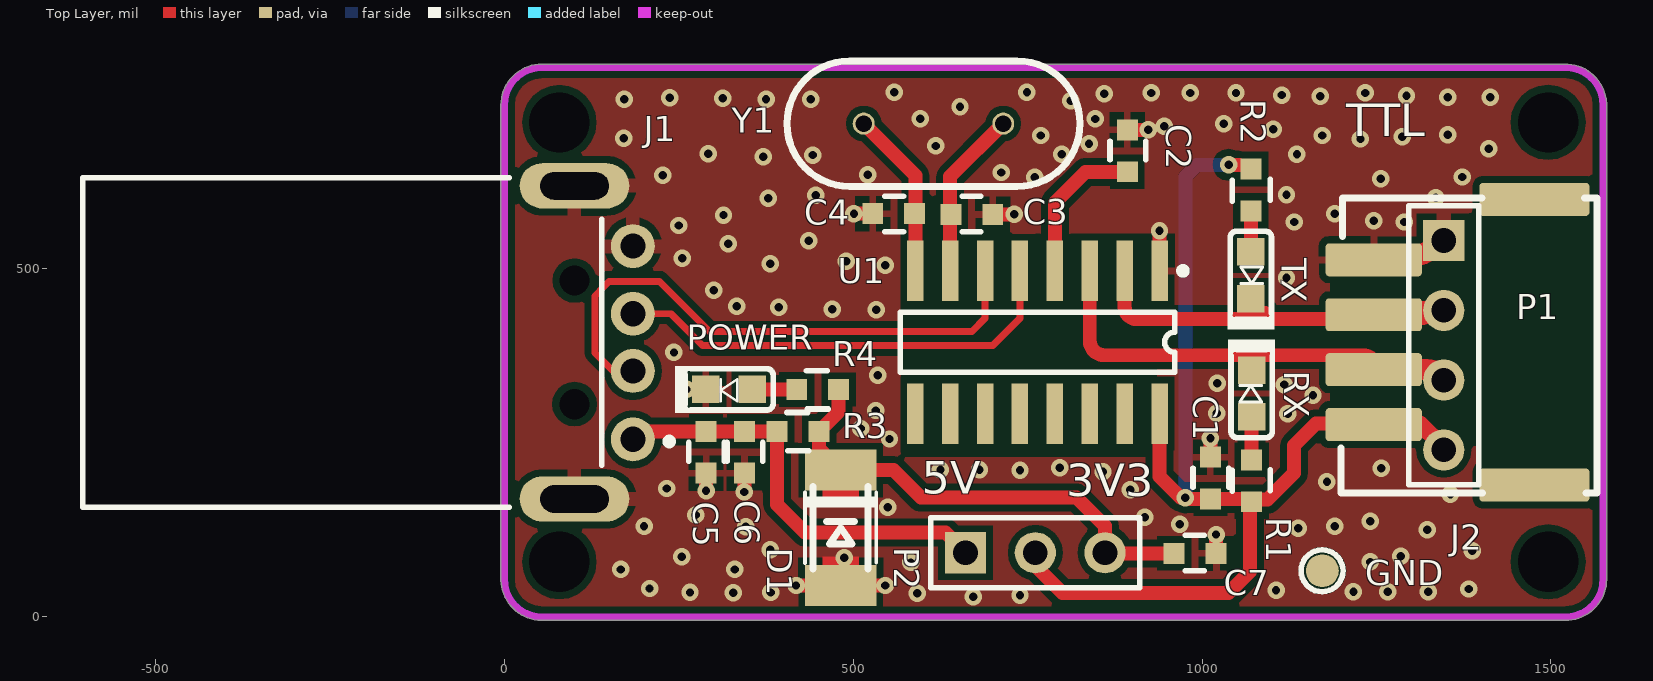
[diagram p0: Top Layer view]
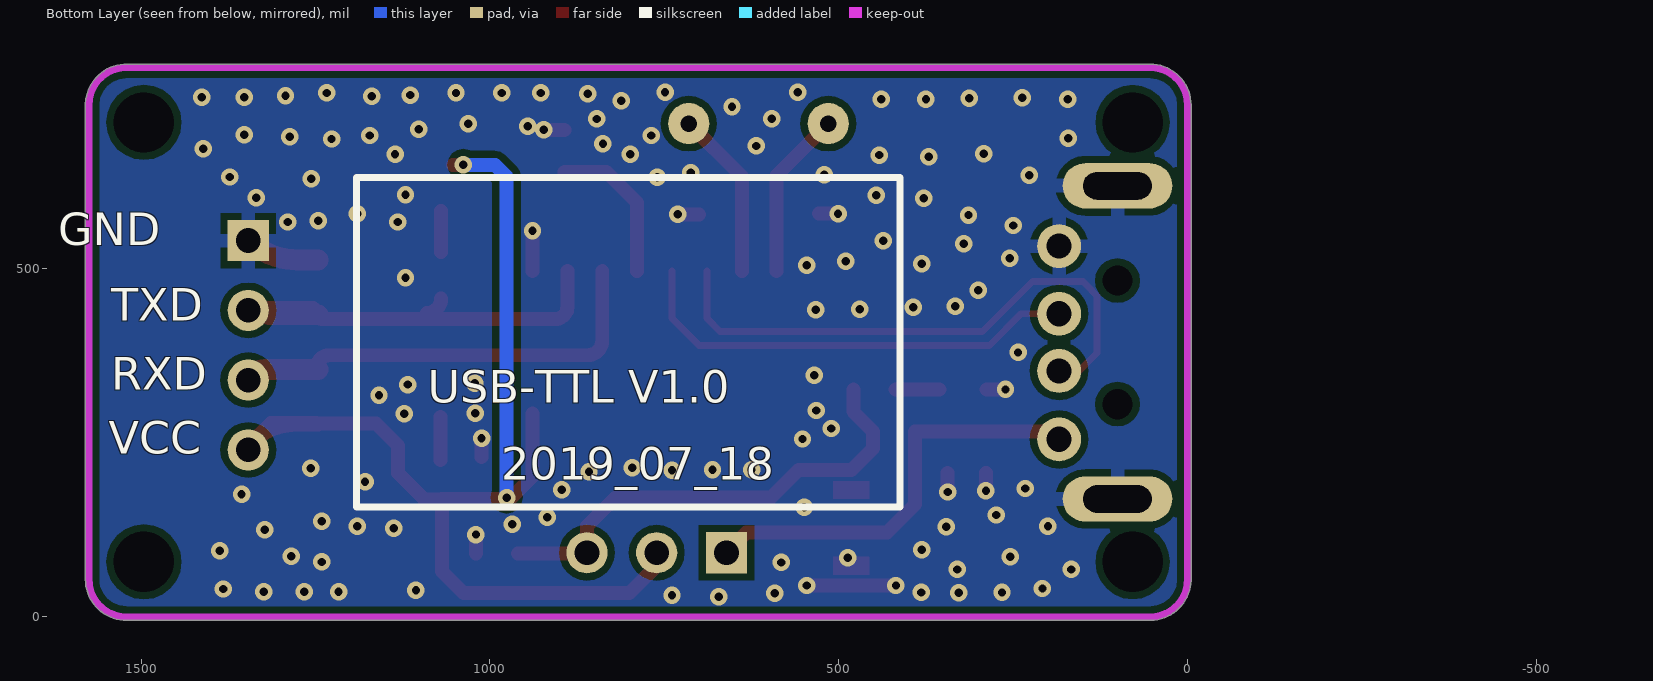
[diagram p1: Bottom Layer view, seen from below]
# Altium PCB MISC50397-29.PcbDoc
Units mil, origin at the board's own origin, x right, y up, seen from the top; angles counter-clockwise.
Board outline 1584.83 x 797.43 mil, 2 copper layers (Top Layer, Bottom Layer), stack 62.249 mil thick; 22 components, 14 nets, 74 pads, 130 vias.

## Layer stack, top to bottom
Top Solder: solder mask 0.4, Solder Resist, Dk 3.5
Top Layer: signal copper 1.4
Dielectric 1: dielectric 59.4488, FR-4, Dk 4.8
Bottom Layer: signal copper 1.4
Bottom Solder: solder mask 0.4, Solder Resist, Dk 3.5

## Board outline
53,-5.01 1520,-5.01 ccw(c1520,0) 1520.4,-5 ccw(c1520.8,0) 1520.8,-5.01 ccw(c1520.8,54) 1579.82,54 ccw(c1574.8,54) 1579.8,54.4 ccw(c1574.8,54.8) 1579.82,54.8 1579.82,736.2 ccw(c1574.8,736.2) 1579.69,737.34 ccw(c1520.8,733.4) 1524.74,792.29 ccw(c1523.6,787.4) 1523.6,792.42 54,792.42 ccw(c54,733.4) -5.01,733.4 -5.01,53 ccw(c0,53) -5,52.59 ccw(c54,54) 52.59,-5 ccw(c53,0)

## Design rules (kind name [scope] priority, off if disabled: settings)
Clearance [All] p1: gap=10 ignorepadtopadclearanceinfootprint=TRUE except(0: Arc-Hole Track-Hole SMDPad-Hole THPad-Hole Via-Hole Fill-Hole Poly-Hole Region-Hole Text-Hole)
PolygonConnect [All] p1: thpad.connectstyle=Relief thpad.reliefconductorwidth=20 thpad.reliefentries=4 thpad.polygonreliefangle="90 Angle" thpad.airgapwidth=10 smdpad.connectstyle=Relief smdpad.reliefconductorwidth=10 smdpad.reliefentries=4 smdpad.polygonreliefangle="90 Angle" smdpad.airgapwidth=10 via.connectstyle=Direct via.reliefconductorwidth=10 via.reliefentries=4 via.polygonreliefangle="90 Angle" via.airgapwidth=10
RoutingVias [All] p1: holewidth=12 width=25 viastyle="Through Hole" minholewidth=12 minwidth=25 maxholewidth=28 maxwidth=50
SolderMaskExpansion [All] p1: expansion=4 istentingtop=FALSE
Width [All] p1: maxlimit=30 minlimit=10 preferedwidth=10
30 further rules are at their usual default settings.

## Components (designator, comment, footprint, x,y, rotation, side; value= is the part's Value field where it differs from the comment)
C1 "0.1uF" CAP0603 1012,169 r90 top
C2 "0.1uF" CAP0603 893,638 r90 top
C3 "22pF" CAP0603 700,577 r180 top
C4 "22pF" CAP0603 528,578 r0 top
C5 "0.1uF" CAP0603 289,206 r90 top
C6 "0.1uF" CAP0603 344,206 r90 top
C7 "0.1uF" CAP0603 1020,91 r180 top
D1 "ZM4733A_C129202" LL-41 482,127.68 r90 top
GND "Comment" TP_T 1172,66 r180 top
J1 "USB-F-HOLE" USB-F-HOLE 177.17,531.5 r270 top locked
J2 "PH2.0/2.54/1.25-SMT-4P" PH2.0-4P-WT 1476.38,598.43 r270 top locked
P1 "Header 4" HDR1X4 1346.46,539.37 r270 top locked
P2 "Header 3" HDR1X3 661,92 r0 top
POWER "LED" LED-0603_RED 322,326 r0 top (schematic designator LED3)
R1 "R" RES0603 1071,225 r270 top
R2 "R" RES0603 1070,582 r90 top
R3 "220R" RES0603 391,266 r0 top
R4 "R" RES0603 419,326 r0 top
RX "LED" LED-0603_RED 1071,320 r270 top (schematic designator LED1)
TX "LED" LED-0603_RED 1070,489.64 r90 top (schematic designator LED2)
U1 "CH340G" SOP16M 764,393.7 r180 top
Y1 "12MHz" XTAL-5.08 515,707 r270 top

## Footprints (in the part's own frame and the unit in brackets; to place one, negate y for a bottom-side part, rotate by r counter-clockwise, add the part's x,y. Pads: shape width x height; smd on the part's side, far side on the other; paste and mask are expansions set on the pad)
CAP0603 [mil] "0603 Capacitor SMD - Startronics"
  rect 30x30 smd: 1(0,0) 2(60,0)
  silkscreen extent 17,-26 44,25, body extent -1,-16 61,16, height 34
HDR1X3 [mm] "Connector; Header; 3 Position"
  rect 1.5x1.5 hole 0.9: 1(0,0)
  round 1.5 hole 0.9: 2(2.54,0) 3(5.08,0)
  silkscreen extent -1.27,-1.27 6.35,1.27
HDR1X4 [mm] "Connector; Header; 4 Position"
  rect 1.5x1.5 hole 0.9: 1(0,0)
  round 1.5 hole 0.9: 2(2.54,0) 3(5.08,0) 4(7.62,0)
  silkscreen extent -1.27,-1.27 8.89,1.27
LED-0603_RED [mm]
  rect 1x1 smd paste+0 mask+0: 1(0.85,0) 2(-0.85,0)
  silkscreen extent -1.97,-0.85 1.6,0.85, body extent -0.92,-0.53 1.09,0.53, height 0.46
LL-41 [mm]
  rect 1.5x2.6 smd: 1(-2.1,0) 2(2.1,0)
  Top Layer region: 1.041,-0.66 1.7,-0.66 1.7,0.66 1.041,0.66
  Top Layer region: -1.727,-0.66 -1.041,-0.66 -1.041,0.66 -1.727,0.66
  silkscreen extent -1.5,-1.3 1.5,1.3, body extent -1.85,-0.81 1.85,0.79, height 1.6
PH2.0-4P-WT [mm]
  rrect20% 1.2x4 smd: 0(0,0) 0(10.4,0)
  rrect20% 1.2x3.5 smd: 1(2.2,-5.85) 2(4.2,-5.85) 3(6.2,-5.85) 4(8.2,-5.85)
  silkscreen extent -0.05,-7.05 10.69,2.29, body extent -0.79,-6.27 11.21,2.13, height 5
RES0603 [mil] "0603 Resistor SMD - Startronics"
  rect 30x30 smd: 1(0,0) 2(60,0)
  silkscreen extent 14,-28 45,27, body extent -2,-16 62,16, height 20
SOP16M [mm]
  rect 0.6x2.2 smd: 1(-4.445,-2.6) 2(-3.175,-2.6) 3(-1.905,-2.6) 4(-0.635,-2.6) 5(0.635,-2.6) 6(1.905,-2.6) 7(3.175,-2.6) 8(4.445,-2.6) 9(4.445,2.6) 10(3.175,2.6) 11(1.905,2.6) 12(0.635,2.6) 13(-0.635,2.6) 14(-1.905,2.6) 15(-3.175,2.6) 16(-4.445,2.6)
  silkscreen extent -5.42,-2.72 5,1.1, body extent -5.15,-3.5 5.15,3.5, height 2.1
TP_T [mm]
  round 1.2 smd: 1(-0.011,-0.004)
  silkscreen extent -0.76,-0.76 0.76,0.76
USB-F-HOLE [mm]
  round 1.6 hole 0.92: 1(7.036,0.178) 2(4.547,0.178) 3(2.464,0.178) 4(0,0.178)
  oval 1.65x4 hole 1 slot 2.5 at 90 deg: 5(-2.195,-1.948) 6(9.205,-1.948)
  round 0.8 hole 1.1 unplated: MH1(1.255,-1.948) MH2(5.755,-1.948)
  silkscreen extent -2.49,-19.85 9.51,1.62, body extent -2.74,-19.65 9.76,0.38, height 3.52
XTAL-5.08 [mm]
  round 0.8 / inner round 0.8 / far side round 1.5 hole 0.6: 1(0,0) 2(0,5.08)
  silkscreen extent -2.29,-2.79 2.29,7.87, body extent -2.26,-2.99 2.24,8.01, height 3.5

## Part data
C1 C2 C3 C4 C5 C6 C7: library part C, BOM_Manufacturer=SEIKO, BOM_Manufacturer Part=XH414HG-IV01E
D1: BOM_Manufacturer="Tak Cheong", BOM_Manufacturer Part=ZM4733A
P1: "Header, 4-Pin"
P2: "Header, 3-Pin"
POWER RX TX: BOM_Manufacturer=EVERLIGHT, BOM_Manufacturer Part=204-10SURD/S530-A3
R1 R2 R4: BOM_Manufacturer Part=?
R3: library part R, BOM_Manufacturer Part=?
U1: "USB2UART"
Y1: library part XTAL

## Free pads (board coordinates)
  rect 19.68x39.37 hole 86.61: 23(78.74,708.66) 24(78.74,78.74) 25(1496.06,708.66) 26(1496.06,78.74)

## Via types
v1: diameter 25/25 (per signal layer), hole 12, Top Layer to Bottom Layer, tented both sides, 118 vias
v2: diameter 25, hole 12, Top Layer to Bottom Layer, tented both sides, 12 vias

## Nets (pads, with @x,y where several pads share a name; then routed paths per layer and width w, separated by ;. In a path a pad name is that pad's centre, name@x,y a point inside that pad or via, vN(x,y) a via of type N, cw(c..) or ccw(c..) an arc to the next point about the centre after c; other vN are vias at no path point)
GND: C1.2 C2.2 C3.1 C4.1 C5.1 C6.1 C7.1 D1.1 J1.4 J1.5 J1.6 J2.1 P1.1 POWER.2 U1.1 | length 518.5
  Top Layer w20: v2(261,326) POWER.2 ; v2(289,181) C5.1 ; v2(344,179) C6.1 ; v2(418,45) D1.1 v2(546,45) ; v2(501,578) C4.1 ; C3.1 v2(731,577) ; C2.2 v2(923,698) ; U1.1 v1(939,553.46) ; C1.2 v2(1012,256) ; C7.1 v2(1020,118)
  Top Layer w30: J2.1 1276.39,511.81 ccw(c1276.39,611.81) 1298.94,514.39 ccw(c1276.39,611.81) 1347.1,541.1 P1.1@1349,543
  other v1: 672,29 739,31 592,34 266,35 328,34.58 382,35 1217,36 1266,36 1324,36 1106,38 1382,40 208,40.72 167,68 330,68 582.58,78 1241,78.74 487,84.53 254,86 1285,86.68 1387,95 381,96 1323,125 1138,126.85 346,129 200.15,130 1190,130 968,133 1241,137 918,143 274,146 549.19,157 1356,176 897,182 232.82,184 1179,193.76 858,208 739,210 625,211 681,211 1257,213 796,214 552,255 511,270 1123,291 1021,292 532,295.84 1159,317.58 1118,333 1021.78,335 535,346.39 243,379 533,440 470,441 393,444 333,445 300,468.41 1121,486 546,504 381,506 490,509.73 255,514 321,535 436,539.03 250,561 1132,566 1290,566 1246,568 314,576 1190,578 378,600 1335,601 446,604.39 1121,604.9 1256,628 760,630 1373,630.51 227,633 521,634 712,637 371,659.76 442,662 799,663 1136,663 292,664 1411,670.94 618,675 838,678 1227,685 171,686 1287,688 769,690 1172,690 1352,691 1102,699 946,703 1031,707 596,714 847,713.72 653,731 812,740 172,742 375,742 439,742 313,743.45 237,744 1352,745 1413,745 1169.5,746 1293,747 1114,748 860,750 927,751 983,751 1048.61,751 1234,751 559,752 749,752
NetC2_1: C2.1 U1.4 | length 220.2
  Top Layer w20: U1.4 788.99,593.99 833,638 C2.1
NetC3_2: C3.2 U1.7 Y1.2 | length 242.4
  Top Layer w20: U1.7 638.99,630.99 Y1.2
NetC4_2: C4.2 U1.8 Y1.1 | length 241.6
  Top Layer w20: Y1.1 588.99,633.01 U1.8
NetJ1_2: J1.2 U1.6 | length 820.8
  Top Layer w10: J1.2 155.5,352.5 130,378 130,459.78 137.12,466.9 137.12,468.12 149.99,480.99 222.01,480.99 294,409 669.99,409 688.99,428 U1.6
NetJ1_3: J1.3 U1.5 | length 657.9
  Top Layer w10: J1.3 238.5,434.5 284,389 699.99,389 738.99,428 U1.5
NetLED1_1: R1.1 RX.1 | length 61.5
  Top Layer w20: R1.1 RX.1
NetLED2_1: R2.1 TX.1 | length 58.9
  Top Layer w20: TX.1 R2.1
NetLED3_1: POWER.1 R4.1 | length 63.5
  Top Layer w20: POWER.1 R4.1
RXD: J2.3 P1.3 RX.2 U1.3 | length 640.6
  Top Layer w20: U1.3 838.99,396.01 ccw(c860,396.01) 860,375 1230.59,375 cw(c1230.59,356.91) 1248.69,356.91 ccw(c1262.59,356.91) J2.3@1248.93,354.33
  Top Layer w30: J2.3 1248.93,354.33 1321.65,354.33 cw(c1321.65,315.65) P1.3@1349,343
TXD: J2.2 P1.2 TX.2 U1.2 | length 640.7
  Top Layer w20: U1.2 888.99,444.01 ccw(c906,444.01) 906,427 1240.04,427 ccw(c1240.04,435.65) 1248.29,433.07 ccw(c1240.04,435.65) 1248.69,435.65 cw(c1256.04,435.65) 1256.04,443 P1.2@1335,443 ; TX.2 ccw(c1090.53,456.17) 1090.53,435.65
  Top Layer w30: J2.2 1248.29,433.07 1311.03,433.07 ccw(c1311.03,466.97) P1.2@1335,443
VCC_3V3: C7.2 D1.2 P2.3 R3.2 R4.2 | length 689.8
  Top Layer w20: R4.2 479,294 R3.2 451,241.36 D1.2 557.64,210.36 597,171 820,171 861,130 P2.3 862,91 C7.2
VCC_5V: C5.2 C6.2 J1.1 P2.1 R3.1 | length 615.2
  Top Layer w20: J1.1 195.67,266 C5.2 C6.2 R3.1 391,161 431,121 632,121 P2.1
VCC_CH340G: C1.1 J2.4 P1.4 P2.2 R1.2 R2.2 U1.16 | length 1708.2
  Top Layer w20: P2.2 761,73 800,34 1038,34 1069,65 R1.2@1069,168 ; U1.16 938.99,201.01 969,171 v2(976,171) 978,169 C1.1 1069,169 R1.2@1069,168 ; v2(1038,648) 1053,648 ; J2.4 1274.99,275.59 cw(c1274.99,175.59) P1.4@1345.7,246.3 ; J2.4@1248.69,277 1163,277 1132,246 1132,206 1094,168 R1.2@1069,168 ; J2.4@1248.69,278.17 1313.83,278.17 P1.4@1345.7,246.3 ; P1.4@1349,243 P1.4@1345.7,246.3
  Bottom Layer w20: v2(976,171) 976,631 993,648 v2(1038,648)
pads on no net: GND.1 J1.MH1 J1.MH2 J2.0 U1.9 U1.10 U1.11 U1.12 U1.13 U1.14 U1.15

## Polygon pours and split planes (outlines as drawn)
GND on Bottom Layer "GND_L02_P002" (solid, remove dead copper, pour order 2): -39.16,716.81 -39.16,818.81 1624.84,818.81 1624.84,-40.19 -34.16,-40.19 -34.16,61.81
GND on Top Layer "GND_L01_P000" (solid, remove dead copper, pour order 0): -56.52,735.75 -56.52,837.75 1607.48,837.75 1607.48,-21.25 -51.52,-21.25 -51.52,80.75

## Keep-outs
Keep-Out Layer:
  lines w10: 0,53 0,733.4 cw(c54,733.4) 54,787.4 1523.6,787.4 ; 0,54 ccw(c54,54) 54,0 ; 53,0 1520,0 ; 1520.8,0 ccw(c1520.8,54) 1574.8,54 ; 1520.8,787.4 cw(c1520.8,733.4) 1574.8,733.4 ; 1574.8,54.8 1574.8,736.2

## Other copper
Top Layer:
  pour cut-out: 1583.48,647.67 1409.01,647.67 1409.01,551.67 1203.48,551.67 1203.48,241.68 1392.94,241.68 1392.94,159.46 1579.69,159.46
  pour cut-out: 567.18,549.37 936,549.37 936,229 568,229 568,249.89

## Silkscreen, mask and mechanical layers (free items; w line width, h text height)
Top Overlay:
  text "TTL" at 1206.34,673 h80
  text "5V" at 598,161 h80
  text "3V3" at 805,157 h80
Bottom Overlay:
  lines w10: 412,157.48 1191,157.48 1191,629.92 412,629.92 412,157.48
  text "GND" at 1619,517 h80
  text "TXD" at 1542.63,409 h80
  text "RXD" at 1542.63,309.5 h80
  text "USB-TTL V1.0" at 1089,291 h80
  text "VCC" at 1546,218 h80
  text "2019_07_18" at 984,181 h80